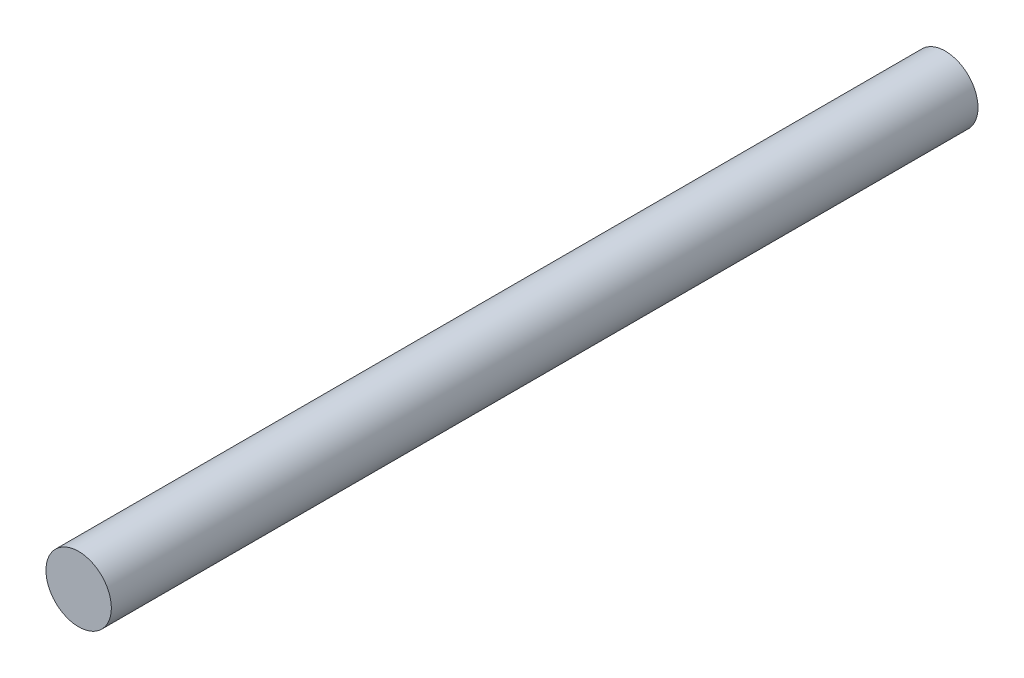
from build123d import *

# Parameters (mm, degrees)
SKETCH_1_R      = 10
EXTRUDE_1_DEPTH = 265


with BuildPart() as part:
    # 草图1 → 凸台-拉伸1 (new body)
    with BuildSketch(Plane.XY):
        Circle(SKETCH_1_R)
    extrude(amount=EXTRUDE_1_DEPTH)


solid = part.part
